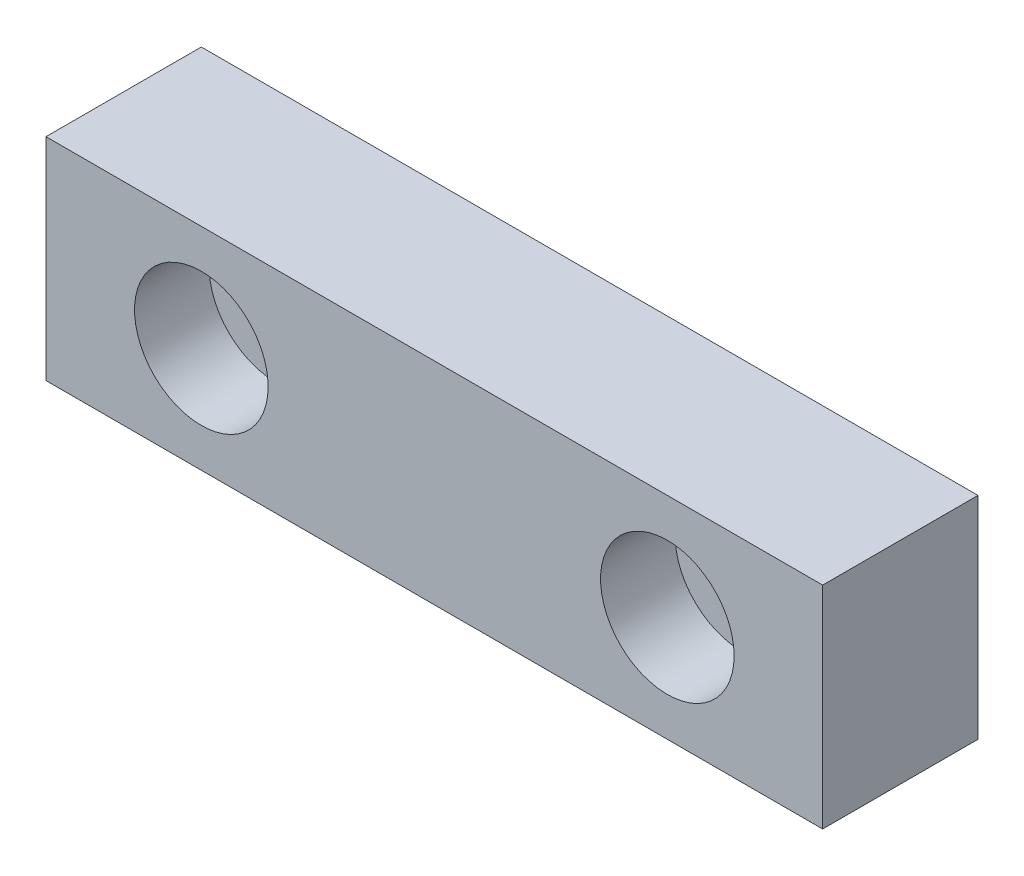
SolidWorks part; units mm, degrees
ref_plane "前视基准面" through (0, 0, 0) normal (0, 0, 1) x (1, 0, 0)
ref_plane "上视基准面" through (0, 0, 0) normal (0, 1, 0) x (1, 0, 0)
ref_plane "右视基准面" through (0, 0, 0) normal (1, 0, 0) x (0, 0, -1)
sketch "草图1" plane through (0, 0, 0) normal (0, 0, 1) x (1, 0, 0)
  line L1 (-8.3455, 3.0394) -> (16.6545, 3.0394)
  line L2 (-8.3455, 3.0394) -> (-8.3455, -3.7606)
  line L3 (-8.3455, -3.7606) -> (16.6545, -3.7606)
  line L4 (16.6545, 3.0394) -> (16.6545, -3.7606)
  dimension "D1" = 6.8
  dimension "D2" = 25
extrude "凸台-拉伸1" add sketch "草图1" along normal blind 5
sketch "草图2" plane through (0, 0, 5) normal (0, 0, 1) x (1, 0, 0)
  line L0 (-8.3455, -3.7606) -> (16.6545, -3.7606) construction
  line L1 (-8.3455, 3.0394) -> (-8.3455, -3.7606) construction
  circle A0 centre (-3.3455, -0.3606) radius 1.2
  circle A1 centre (11.6545, -0.3606) radius 1.2
  dimension "D1" = 2.4
  dimension "D2" = 2.4
  dimension "D3" = 3.4
  dimension "D4" = 5
  dimension "D5" = 15
  dimension "D6" = 3.4
extrude "切除-拉伸1" cut sketch "草图2" against normal up to next
sketch "草图3" plane through (0, 0, 5) normal (0, 0, 1) x (1, 0, 0)
  circle A0 centre (-3.3455, -0.3606) radius 2.15
  circle A1 centre (11.6545, -0.3606) radius 2.15
  dimension "D1" = 4.3
  dimension "D2" = 2
extrude "切除-拉伸2" cut sketch "草图3" against normal blind 2.4
